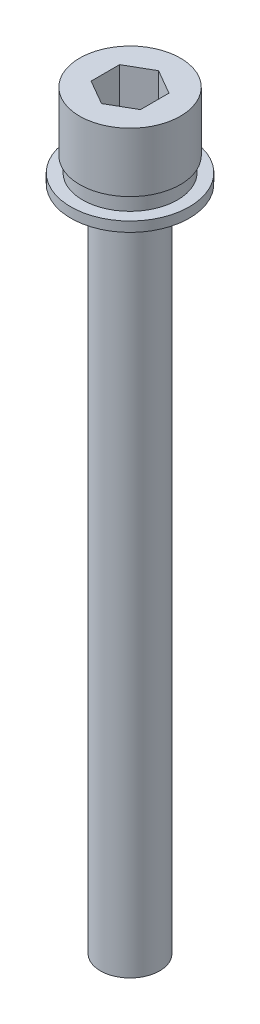
from build123d import *

# Parameters (mm, degrees)
CUT_EXTRUDE_1_DEPTH  = 5
SKETCH_3_R           = 4.8
SKETCH_3_R_2         = 3
BOSS_EXTRUDE_1_DEPTH = 1.5
SKETCH_4_R           = 6
SKETCH_4_R_2         = 3
BOSS_EXTRUDE_2_DEPTH = 1


with BuildPart() as part:
    # Sketch 1 → Revolve 1 (revolve)
    with BuildSketch(Plane.XY, mode=Mode.PRIVATE) as revolve_1_sk:
        Polygon((0, 6), (-5.1, 6), (-5.1, 0), (-3, 0), (-3, -70), (0, -70), align=None)
    revolve(revolve_1_sk.sketch.rotate(Axis((0, 11.322033898, 0), (0, -1, 0)), 270), axis=Axis((0, 11.322033898, 0), (0, -1, 0)))

    # Sketch 2 → Cut-Extrude 1 (cut)
    with BuildSketch(Plane(origin=(0, 6, 0), x_dir=(1, 0, 0), z_dir=(0, 1, 0))):
        Polygon((0, 2.886751346), (-2.5, 1.443375673), (-2.5, -1.443375673), (0, -2.886751346), (2.5, -1.443375673), (2.5, 1.443375673), align=None)
    extrude(amount=-CUT_EXTRUDE_1_DEPTH, mode=Mode.SUBTRACT)


with BuildPart() as body_2:
    # Sketch 3 → Boss-Extrude 1 (new body)
    with BuildSketch(Plane.XZ):
        with Locations(Location((0, 0, 0), (0, 0, 270))):
            Circle(SKETCH_3_R)
        with Locations(Location((0, 0, 0), (0, 0, 270))):
            Circle(SKETCH_3_R_2, mode=Mode.SUBTRACT)
    extrude(amount=BOSS_EXTRUDE_1_DEPTH)


with BuildPart() as body_3:
    # Sketch 4 → Boss-Extrude 2 (new body)
    with BuildSketch(Plane.XZ.offset(1.5)):
        with Locations(Location((0, 0, 0), (0, 0, 270))):
            Circle(SKETCH_4_R)
        with Locations(Location((0, 0, 0), (0, 0, 270))):
            Circle(SKETCH_4_R_2, mode=Mode.SUBTRACT)
    extrude(amount=BOSS_EXTRUDE_2_DEPTH)


solid = Compound([part.part, body_2.part, body_3.part])
